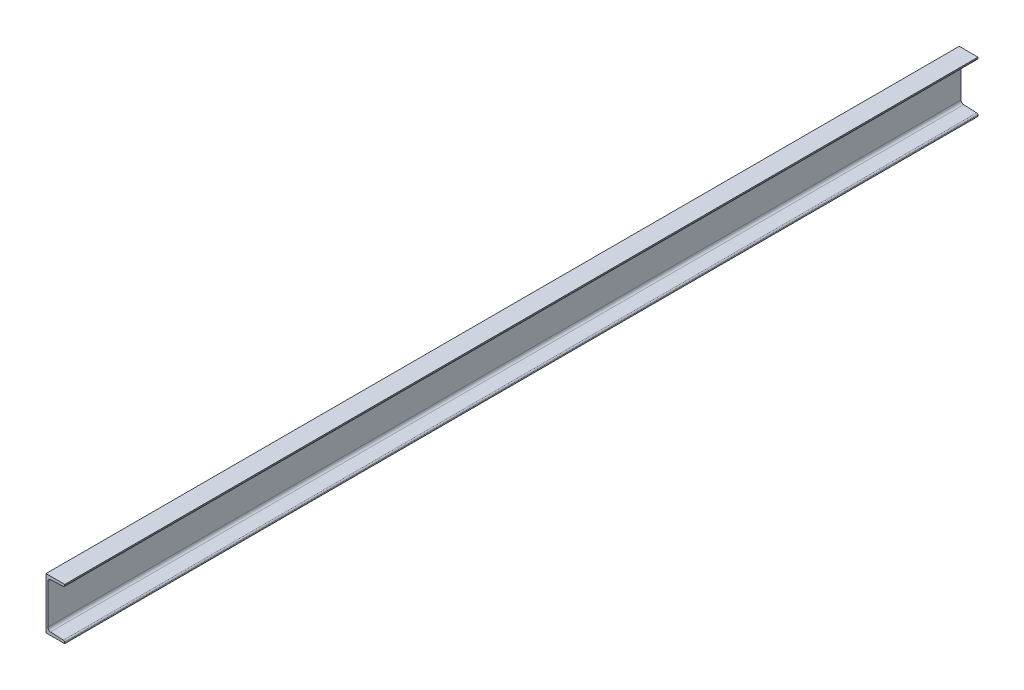
from build123d import *

# Parameters (mm, degrees)
BOSS_EXTRUDE1_DEPTH = 1778


with BuildPart() as part:
    # Sketch1 → Boss-Extrude1 (new, symmetric)
    with BuildSketch(Plane(origin=(28.211262136, 0, 0), x_dir=(-1, 0, 0), z_dir=(0, 0, 1))):
        with BuildLine():
            Line((28.211262136, 0), (28.211262136, -200))
            Line((28.211262136, -200), (-44.788737864, -200))
            Line((-44.788737864, -200), (-44.788737864, -196.033179359))
            ThreePointArc((-44.788737864, -196.033179359), (-43.272315441, -192.240936001), (-39.559243433, -190.539835501))
            Line((-39.559243433, -190.539835501), (10.752273273, -188.062374452))
            ThreePointArc((10.752273273, -188.062374452), (18.17841729, -184.660173452), (21.211262136, -177.075686736))
            Line((21.211262136, -177.075686736), (21.211262136, -22.924313264))
            ThreePointArc((21.211262136, -22.924313264), (18.17841729, -15.339826548), (10.752273273, -11.937625548))
            Line((10.752273273, -11.937625548), (-39.559243433, -9.460164499))
            ThreePointArc((-39.559243433, -9.460164499), (-43.272315441, -7.759063999), (-44.788737864, -3.966820641))
            Line((-44.788737864, -3.966820641), (-44.788737864, 0))
            Line((-44.788737864, 0), (28.211262136, 0))
        make_face()
    extrude(amount=BOSS_EXTRUDE1_DEPTH, both=True)


solid = part.part
